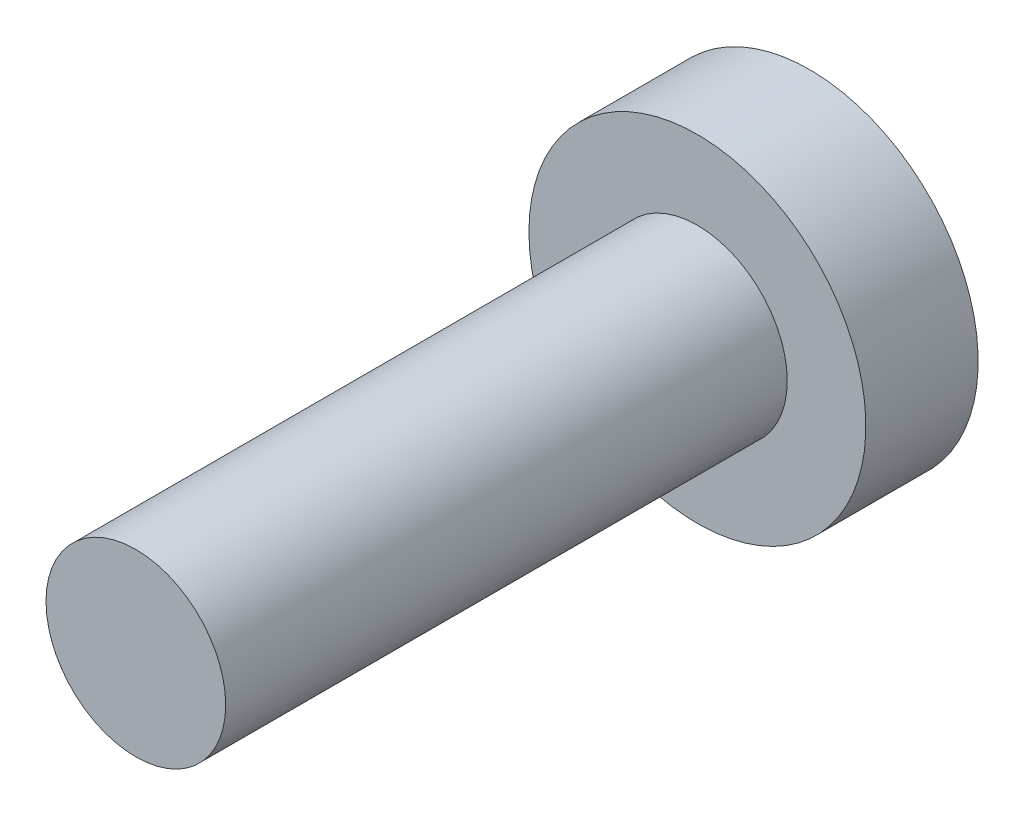
SolidWorks part; units mm, degrees
material "45"
ref_plane "Front" through (0, 0, 0) normal (0, 0, 1) x (1, 0, 0)
ref_plane "Top" through (0, 0, 0) normal (0, 1, 0) x (1, 0, 0)
ref_plane "Right" through (0, 0, 0) normal (1, 0, 0) x (0, 0, -1)
sketch "Sketch1" plane through (0, 0, 0) normal (0, 0, 1) x (1, 0, 0)
  circle A0 centre (0, 0) radius 4
  dimension "D1" = 8
extrude "Boss-Extrude1" add sketch "Sketch1" along normal blind 25
sketch "Sketch2" plane through (0, 0, 0) normal (0, 0, -1) x (-1, 0, 0)
  circle A0 centre (0, 0) radius 7.5
  dimension "D1" = 15
extrude "Boss-Extrude2" add sketch "Sketch2" along normal blind 5
equation "\"零件重量\"= IIF ( \"SW-质量\" > 100 , int ( \"SW-质量\" ) , \"SW-质量\" )"
